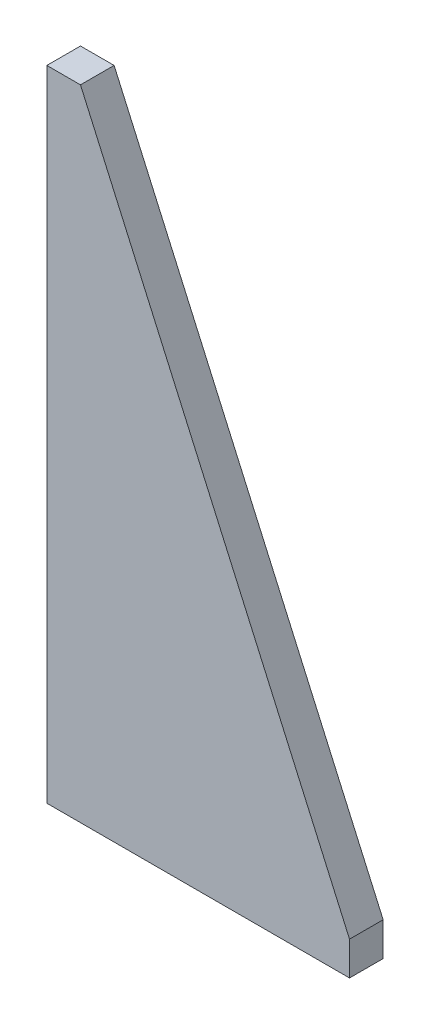
from build123d import *

# Parameters (mm, degrees)
BOSS_EXTRUDE1_DEPTH = 10


with BuildPart() as part:
    # Sketch1 → Boss-Extrude1 (new body)
    with BuildSketch(Plane.XY):
        Polygon((0, 0), (90, 0), (90, 10), (10, 190), (0, 190), align=None)
    extrude(amount=BOSS_EXTRUDE1_DEPTH)


solid = part.part
